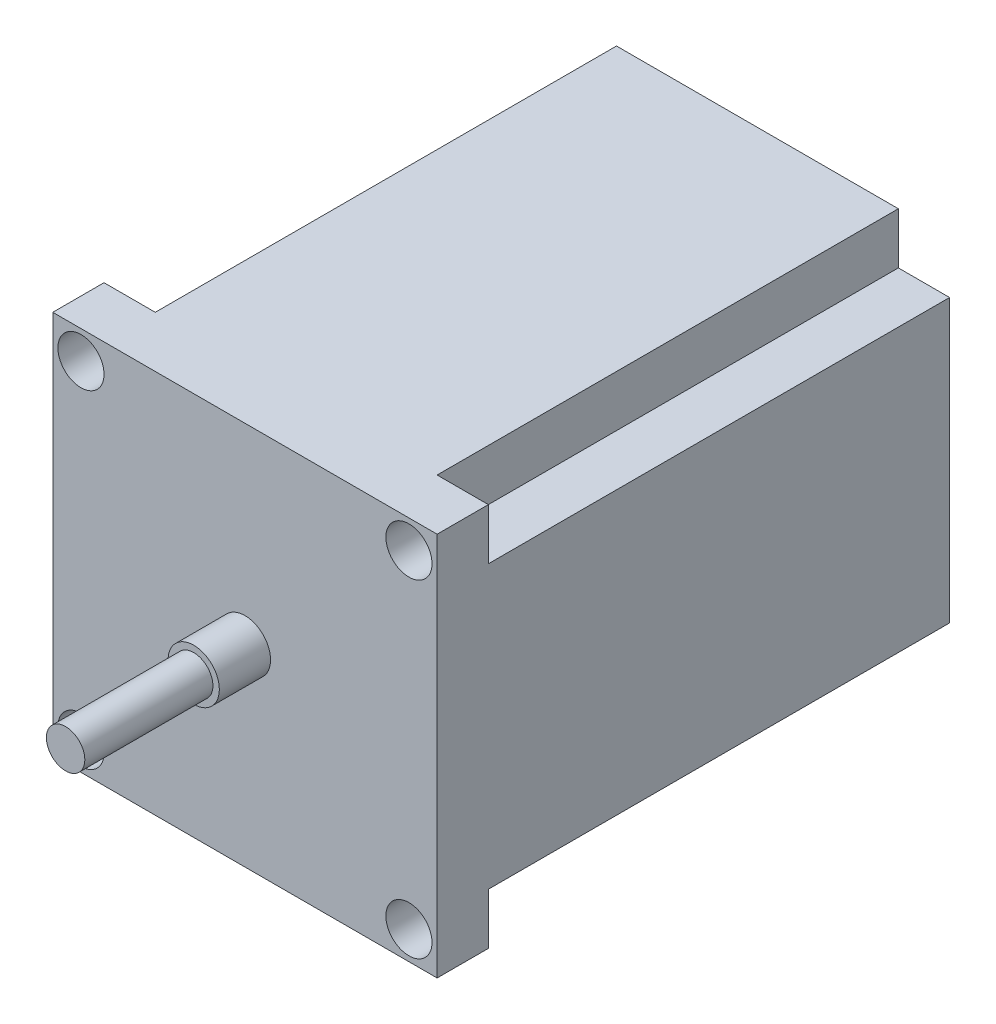
from build123d import *

# Parameters (mm, degrees)
SKETCH1_W           = 15
SKETCH1_H           = 15
BOSS_EXTRUDE1_DEPTH = 20
SKETCH5_W           = 2
SKETCH5_H           = 2
CUT_EXTRUDE1_DEPTH  = 18
SKETCH2_R           = 0.9
CUT_EXTRUDE2_DEPTH  = 71
SKETCH6_R           = 1
BOSS_EXTRUDE2_DEPTH = 2
SKETCH7_R           = 0.75
BOSS_EXTRUDE3_DEPTH = 5


with BuildPart() as part:
    # Sketch1 → Boss-Extrude1 (new body)
    with BuildSketch(Plane.XY):
        Rectangle(SKETCH1_W, SKETCH1_H)
    extrude(amount=BOSS_EXTRUDE1_DEPTH)

    # Sketch5 → Cut-Extrude1 (cut)
    with BuildSketch(Plane(origin=(0, 0, 0), x_dir=(-1, 0, 0), z_dir=(0, 0, -1))):
        with Locations((6.5, 6.5)):
            Rectangle(SKETCH5_W, SKETCH5_H)
        with Locations((6.5, -6.5)):
            Rectangle(SKETCH5_W, SKETCH5_H)
        with Locations((-6.5, -6.5)):
            Rectangle(SKETCH5_W, SKETCH5_H)
        with Locations((-6.5, 6.5)):
            Rectangle(SKETCH5_W, SKETCH5_H)
    extrude(amount=-CUT_EXTRUDE1_DEPTH, mode=Mode.SUBTRACT)

    # Sketch2 → Cut-Extrude2 (cut)
    with BuildSketch(Plane.XY.offset(20)):
        with Locations((6.4, 6.4)):
            Circle(SKETCH2_R)
        with Locations((-6.4, 6.4)):
            Circle(SKETCH2_R)
        with Locations((-6.4, -6.4)):
            Circle(SKETCH2_R)
        with Locations((6.4, -6.4)):
            Circle(SKETCH2_R)
    extrude(amount=-CUT_EXTRUDE2_DEPTH, mode=Mode.SUBTRACT)

    # Sketch6 → Boss-Extrude2 (add)
    with BuildSketch(Plane.XY.offset(20)):
        with Locations(Location((0, 0, 0), (0, 0, 180))):
            Circle(SKETCH6_R)
    extrude(amount=BOSS_EXTRUDE2_DEPTH)

    # Sketch7 → Boss-Extrude3 (add)
    with BuildSketch(Plane.XY.offset(22)):
        Circle(SKETCH7_R)
    extrude(amount=BOSS_EXTRUDE3_DEPTH)


solid = part.part
